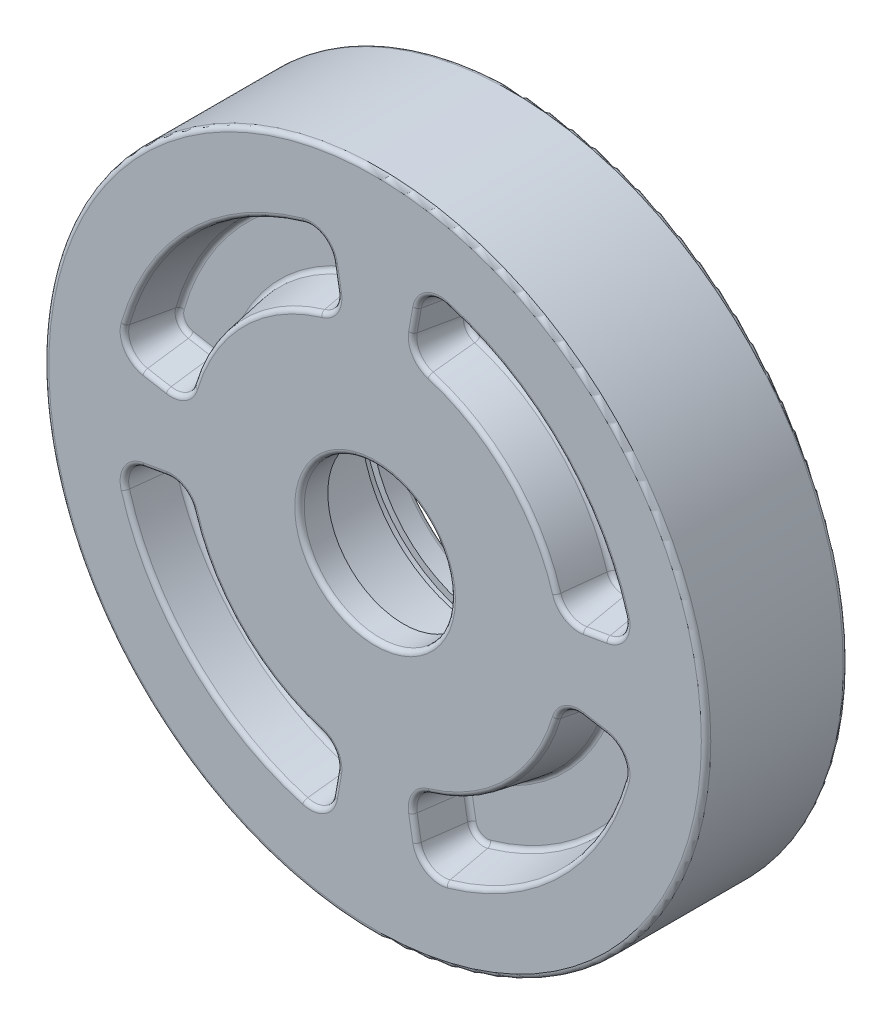
from build123d import *

# Parameters (mm, degrees)
SKETCH1_R                = 70
BOSS_EXTRUDE1_DEPTH      = 15
SKETCH2_R                = 16
CUT_EXTRUDE1_DEPTH       = 6
SKETCH3_R                = 22.5
CUT_EXTRUDE2_DEPTH       = 2
SKETCH4_R                = 26
CUT_EXTRUDE3_DEPTH       = 15
SKETCH5_R                = 27.5
CUT_EXTRUDE4_DEPTH       = 2
SKETCH6_R                = 26
CUT_EXTRUDE5_DEPTH       = 103.102889283
CUT_EXTRUDE6_DEPTH       = 10
CUT_EXTRUDE6_DRAFT       = -10
CIRPATTERN1_COPY_1_DEPTH = 10
CIRPATTERN1_COPY_1_DRAFT = -10
CIRPATTERN1_COPY_2_DEPTH = 10
CIRPATTERN1_COPY_2_DRAFT = -10
CIRPATTERN1_COPY_3_DEPTH = 10
CIRPATTERN1_COPY_3_DRAFT = -10
MIRROR1_COPY_1_DEPTH     = 10
MIRROR1_COPY_1_DRAFT     = -10
MIRROR1_COPY_2_DEPTH     = 10
MIRROR1_COPY_2_DRAFT     = -10
MIRROR1_COPY_3_DEPTH     = 10
MIRROR1_COPY_3_DRAFT     = -10
MIRROR1_COPY_4_DEPTH     = 10
MIRROR1_COPY_4_DRAFT     = -10
FILLET1_R                = 1
FILLET2_R                = 1
SKETCH8_R                = 1.5
CUT_EXTRUDE7_DEPTH       = 10


with BuildPart() as part:
    # Sketch1 → Boss-Extrude1 (new, symmetric)
    with BuildSketch(Plane.XY):
        Circle(SKETCH1_R)
    extrude(amount=BOSS_EXTRUDE1_DEPTH, both=True)

    # Sketch2 → Cut-Extrude1 (cut)
    with BuildSketch(Plane.XY.offset(15)):
        Circle(SKETCH2_R)
    extrude(amount=-CUT_EXTRUDE1_DEPTH, mode=Mode.SUBTRACT)

    # Sketch3 → Cut-Extrude2 (cut)
    with BuildSketch(Plane.XY.offset(9)):
        Circle(SKETCH3_R)
    extrude(amount=-CUT_EXTRUDE2_DEPTH, mode=Mode.SUBTRACT)

    # Sketch4 → Cut-Extrude3 (cut)
    with BuildSketch(Plane.XY.offset(7)):
        Circle(SKETCH4_R)
    extrude(amount=-CUT_EXTRUDE3_DEPTH, mode=Mode.SUBTRACT)

    # Sketch5 → Cut-Extrude4 (cut)
    with BuildSketch(Plane.XY.offset(-8)):
        Circle(SKETCH5_R)
    extrude(amount=-CUT_EXTRUDE4_DEPTH, mode=Mode.SUBTRACT)

    # Sketch6 → Cut-Extrude5 (cut, through all)
    with BuildSketch(Plane.XY.offset(-10)):
        Circle(SKETCH6_R)
    extrude(amount=-CUT_EXTRUDE5_DEPTH, mode=Mode.SUBTRACT)


with BuildPart() as cut_extrude6_tool:
    # Sketch7 → Cut-Extrude6 (with draft: the straight prism first)
    with BuildSketch(Plane(origin=(0, 0, -15), x_dir=(-1, 0, 0), z_dir=(0, 0, -1))):
        with BuildLine():
            ThreePointArc((-8.800542906, 48.942287572), (-11.071183936, 52.316508785), (-15.098039216, 52.887136544))
            ThreePointArc((-15.098039216, 52.887136544), (-38.890872965, 38.890872965), (-52.887136544, 15.098039216))
            ThreePointArc((-52.887136544, 15.098039216), (-52.316508785, 11.071183936), (-48.942287572, 8.800542906))
            Line((-48.942287572, 8.800542906), (-43.987240669, 7.932195568))
            ThreePointArc((-43.987240669, 7.932195568), (-40.494635393, 8.60443107), (-38.3325939, 11.428571429))
            ThreePointArc((-38.3325939, 11.428571429), (-28.284271247, 28.284271247), (-11.428571429, 38.3325939))
            ThreePointArc((-11.428571429, 38.3325939), (-8.60443107, 40.494635393), (-7.932195568, 43.987240669))
            Line((-7.932195568, 43.987240669), (-8.800542906, 48.942287572))
        make_face()
    extrude(amount=-CUT_EXTRUDE6_DEPTH)
    # Cut-Extrude6: the draft: its side faces are tilted about the plane it starts from
    cut_extrude6_sides = [cut_extrude6_tool.faces().sort_by_distance(p)[0] for p in [
        (8.60443107, 40.494635393, -10),
        (8.366369237, 46.46476412, -10),
        (11.071183936, 52.316508785, -10),
        (38.890872965, 38.890872965, -10),
        (52.316508785, 11.071183936, -10),
        (46.46476412, 8.366369237, -10),
        (40.494635393, 8.60443107, -10),
        (28.284271247, 28.284271247, -10),
    ]]
    draft(cut_extrude6_sides, Plane(origin=(0, 0, -15), x_dir=(-1, 0, 0), z_dir=(0, 0, -1)), CUT_EXTRUDE6_DRAFT)


with BuildPart() as part_1:
    add(part.part)

    # Cut-Extrude6: cut by cut_extrude6_tool
    add(cut_extrude6_tool.part, mode=Mode.SUBTRACT)


with BuildPart() as cirpattern1_copy_1_tool:
    # CirPattern1 copy 1 sketch → CirPattern1 copy 1 (with draft: the straight prism first)
    with BuildSketch(Plane(origin=(0, 0, -15), x_dir=(0, -1, 0), z_dir=(0, 0, -1))):
        with BuildLine():
            ThreePointArc((-8.800542906, 48.942287572), (-11.071183936, 52.316508785), (-15.098039216, 52.887136544))
            ThreePointArc((-15.098039216, 52.887136544), (-38.890872965, 38.890872965), (-52.887136544, 15.098039216))
            ThreePointArc((-52.887136544, 15.098039216), (-52.316508785, 11.071183936), (-48.942287572, 8.800542906))
            Line((-48.942287572, 8.800542906), (-43.987240669, 7.932195568))
            ThreePointArc((-43.987240669, 7.932195568), (-40.494635393, 8.60443107), (-38.3325939, 11.428571429))
            ThreePointArc((-38.3325939, 11.428571429), (-28.284271247, 28.284271247), (-11.428571429, 38.3325939))
            ThreePointArc((-11.428571429, 38.3325939), (-8.60443107, 40.494635393), (-7.932195568, 43.987240669))
            Line((-7.932195568, 43.987240669), (-8.800542906, 48.942287572))
        make_face()
    extrude(amount=-CIRPATTERN1_COPY_1_DEPTH)
    # CirPattern1 copy 1: the draft: its side faces are tilted about the plane it starts from
    cirpattern1_copy_1_sides = [cirpattern1_copy_1_tool.faces().sort_by_distance(p)[0] for p in [
        (-40.494635393, 8.60443107, -10),
        (-46.46476412, 8.366369237, -10),
        (-52.316508785, 11.071183936, -10),
        (-38.890872965, 38.890872965, -10),
        (-11.071183936, 52.316508785, -10),
        (-8.366369237, 46.46476412, -10),
        (-8.60443107, 40.494635393, -10),
        (-28.284271247, 28.284271247, -10),
    ]]
    draft(cirpattern1_copy_1_sides, Plane(origin=(0, 0, -15), x_dir=(0, -1, 0), z_dir=(0, 0, -1)), CIRPATTERN1_COPY_1_DRAFT)


with BuildPart() as part_2:
    add(part_1.part)

    # CirPattern1 copy 1: cut by cirpattern1_copy_1_tool
    add(cirpattern1_copy_1_tool.part, mode=Mode.SUBTRACT)


with BuildPart() as cirpattern1_copy_2_tool:
    # CirPattern1 copy 2 sketch → CirPattern1 copy 2 (with draft: the straight prism first)
    with BuildSketch(Plane(origin=(0, 0, -15), x_dir=(1, 0, 0), z_dir=(0, 0, -1))):
        with BuildLine():
            ThreePointArc((-8.800542906, 48.942287572), (-11.071183936, 52.316508785), (-15.098039216, 52.887136544))
            ThreePointArc((-15.098039216, 52.887136544), (-38.890872965, 38.890872965), (-52.887136544, 15.098039216))
            ThreePointArc((-52.887136544, 15.098039216), (-52.316508785, 11.071183936), (-48.942287572, 8.800542906))
            Line((-48.942287572, 8.800542906), (-43.987240669, 7.932195568))
            ThreePointArc((-43.987240669, 7.932195568), (-40.494635393, 8.60443107), (-38.3325939, 11.428571429))
            ThreePointArc((-38.3325939, 11.428571429), (-28.284271247, 28.284271247), (-11.428571429, 38.3325939))
            ThreePointArc((-11.428571429, 38.3325939), (-8.60443107, 40.494635393), (-7.932195568, 43.987240669))
            Line((-7.932195568, 43.987240669), (-8.800542906, 48.942287572))
        make_face()
    extrude(amount=-CIRPATTERN1_COPY_2_DEPTH)
    # CirPattern1 copy 2: the draft: its side faces are tilted about the plane it starts from
    cirpattern1_copy_2_sides = [cirpattern1_copy_2_tool.faces().sort_by_distance(p)[0] for p in [
        (-8.60443107, -40.494635393, -10),
        (-8.366369237, -46.46476412, -10),
        (-11.071183936, -52.316508785, -10),
        (-38.890872965, -38.890872965, -10),
        (-52.316508785, -11.071183936, -10),
        (-46.46476412, -8.366369237, -10),
        (-40.494635393, -8.60443107, -10),
        (-28.284271247, -28.284271247, -10),
    ]]
    draft(cirpattern1_copy_2_sides, Plane(origin=(0, 0, -15), x_dir=(1, 0, 0), z_dir=(0, 0, -1)), CIRPATTERN1_COPY_2_DRAFT)


with BuildPart() as part_3:
    add(part_2.part)

    # CirPattern1 copy 2: cut by cirpattern1_copy_2_tool
    add(cirpattern1_copy_2_tool.part, mode=Mode.SUBTRACT)


with BuildPart() as cirpattern1_copy_3_tool:
    # CirPattern1 copy 3 sketch → CirPattern1 copy 3 (with draft: the straight prism first)
    with BuildSketch(Plane.YX.offset(15)):
        with BuildLine():
            ThreePointArc((-8.800542906, 48.942287572), (-11.071183936, 52.316508785), (-15.098039216, 52.887136544))
            ThreePointArc((-15.098039216, 52.887136544), (-38.890872965, 38.890872965), (-52.887136544, 15.098039216))
            ThreePointArc((-52.887136544, 15.098039216), (-52.316508785, 11.071183936), (-48.942287572, 8.800542906))
            Line((-48.942287572, 8.800542906), (-43.987240669, 7.932195568))
            ThreePointArc((-43.987240669, 7.932195568), (-40.494635393, 8.60443107), (-38.3325939, 11.428571429))
            ThreePointArc((-38.3325939, 11.428571429), (-28.284271247, 28.284271247), (-11.428571429, 38.3325939))
            ThreePointArc((-11.428571429, 38.3325939), (-8.60443107, 40.494635393), (-7.932195568, 43.987240669))
            Line((-7.932195568, 43.987240669), (-8.800542906, 48.942287572))
        make_face()
    extrude(amount=-CIRPATTERN1_COPY_3_DEPTH)
    # CirPattern1 copy 3: the draft: its side faces are tilted about the plane it starts from
    cirpattern1_copy_3_sides = [cirpattern1_copy_3_tool.faces().sort_by_distance(p)[0] for p in [
        (40.494635393, -8.60443107, -10),
        (46.46476412, -8.366369237, -10),
        (52.316508785, -11.071183936, -10),
        (38.890872965, -38.890872965, -10),
        (11.071183936, -52.316508785, -10),
        (8.366369237, -46.46476412, -10),
        (8.60443107, -40.494635393, -10),
        (28.284271247, -28.284271247, -10),
    ]]
    draft(cirpattern1_copy_3_sides, Plane.YX.offset(15), CIRPATTERN1_COPY_3_DRAFT)


with BuildPart() as part_4:
    add(part_3.part)

    # CirPattern1 copy 3: cut by cirpattern1_copy_3_tool
    add(cirpattern1_copy_3_tool.part, mode=Mode.SUBTRACT)


with BuildPart() as mirror1_copy_1_tool:
    # Mirror1 copy 1 sketch → Mirror1 copy 1 (with draft: the straight prism first)
    with BuildSketch(Plane(origin=(0, 0, 15), x_dir=(-1, 0, 0), z_dir=(0, 0, 1))):
        with BuildLine():
            ThreePointArc((-8.800542906, -48.942287572), (-11.071183936, -52.316508785), (-15.098039216, -52.887136544))
            ThreePointArc((-15.098039216, -52.887136544), (-38.890872965, -38.890872965), (-52.887136544, -15.098039216))
            ThreePointArc((-52.887136544, -15.098039216), (-52.316508785, -11.071183936), (-48.942287572, -8.800542906))
            Line((-48.942287572, -8.800542906), (-43.987240669, -7.932195568))
            ThreePointArc((-43.987240669, -7.932195568), (-40.494635393, -8.60443107), (-38.3325939, -11.428571429))
            ThreePointArc((-38.3325939, -11.428571429), (-28.284271247, -28.284271247), (-11.428571429, -38.3325939))
            ThreePointArc((-11.428571429, -38.3325939), (-8.60443107, -40.494635393), (-7.932195568, -43.987240669))
            Line((-7.932195568, -43.987240669), (-8.800542906, -48.942287572))
        make_face()
    extrude(amount=-MIRROR1_COPY_1_DEPTH)
    # Mirror1 copy 1: the draft: its side faces are tilted about the plane it starts from
    mirror1_copy_1_sides = [mirror1_copy_1_tool.faces().sort_by_distance(p)[0] for p in [
        (8.60443107, 40.494635393, 10),
        (8.366369237, 46.46476412, 10),
        (11.071183936, 52.316508785, 10),
        (38.890872965, 38.890872965, 10),
        (52.316508785, 11.071183936, 10),
        (46.46476412, 8.366369237, 10),
        (40.494635393, 8.60443107, 10),
        (28.284271247, 28.284271247, 10),
    ]]
    draft(mirror1_copy_1_sides, Plane(origin=(0, 0, 15), x_dir=(-1, 0, 0), z_dir=(0, 0, 1)), MIRROR1_COPY_1_DRAFT)


with BuildPart() as part_5:
    add(part_4.part)

    # Mirror1 copy 1: cut by mirror1_copy_1_tool
    add(mirror1_copy_1_tool.part, mode=Mode.SUBTRACT)


with BuildPart() as mirror1_copy_2_tool:
    # Mirror1 copy 2 sketch → Mirror1 copy 2 (with draft: the straight prism first)
    with BuildSketch(Plane(origin=(0, 0, 15), x_dir=(0, -1, 0), z_dir=(0, 0, 1))):
        with BuildLine():
            ThreePointArc((-8.800542906, -48.942287572), (-11.071183936, -52.316508785), (-15.098039216, -52.887136544))
            ThreePointArc((-15.098039216, -52.887136544), (-38.890872965, -38.890872965), (-52.887136544, -15.098039216))
            ThreePointArc((-52.887136544, -15.098039216), (-52.316508785, -11.071183936), (-48.942287572, -8.800542906))
            Line((-48.942287572, -8.800542906), (-43.987240669, -7.932195568))
            ThreePointArc((-43.987240669, -7.932195568), (-40.494635393, -8.60443107), (-38.3325939, -11.428571429))
            ThreePointArc((-38.3325939, -11.428571429), (-28.284271247, -28.284271247), (-11.428571429, -38.3325939))
            ThreePointArc((-11.428571429, -38.3325939), (-8.60443107, -40.494635393), (-7.932195568, -43.987240669))
            Line((-7.932195568, -43.987240669), (-8.800542906, -48.942287572))
        make_face()
    extrude(amount=-MIRROR1_COPY_2_DEPTH)
    # Mirror1 copy 2: the draft: its side faces are tilted about the plane it starts from
    mirror1_copy_2_sides = [mirror1_copy_2_tool.faces().sort_by_distance(p)[0] for p in [
        (-40.494635393, 8.60443107, 10),
        (-46.46476412, 8.366369237, 10),
        (-52.316508785, 11.071183936, 10),
        (-38.890872965, 38.890872965, 10),
        (-11.071183936, 52.316508785, 10),
        (-8.366369237, 46.46476412, 10),
        (-8.60443107, 40.494635393, 10),
        (-28.284271247, 28.284271247, 10),
    ]]
    draft(mirror1_copy_2_sides, Plane(origin=(0, 0, 15), x_dir=(0, -1, 0), z_dir=(0, 0, 1)), MIRROR1_COPY_2_DRAFT)


with BuildPart() as part_6:
    add(part_5.part)

    # Mirror1 copy 2: cut by mirror1_copy_2_tool
    add(mirror1_copy_2_tool.part, mode=Mode.SUBTRACT)


with BuildPart() as mirror1_copy_3_tool:
    # Mirror1 copy 3 sketch → Mirror1 copy 3 (with draft: the straight prism first)
    with BuildSketch(Plane.XY.offset(15)):
        with BuildLine():
            ThreePointArc((-8.800542906, -48.942287572), (-11.071183936, -52.316508785), (-15.098039216, -52.887136544))
            ThreePointArc((-15.098039216, -52.887136544), (-38.890872965, -38.890872965), (-52.887136544, -15.098039216))
            ThreePointArc((-52.887136544, -15.098039216), (-52.316508785, -11.071183936), (-48.942287572, -8.800542906))
            Line((-48.942287572, -8.800542906), (-43.987240669, -7.932195568))
            ThreePointArc((-43.987240669, -7.932195568), (-40.494635393, -8.60443107), (-38.3325939, -11.428571429))
            ThreePointArc((-38.3325939, -11.428571429), (-28.284271247, -28.284271247), (-11.428571429, -38.3325939))
            ThreePointArc((-11.428571429, -38.3325939), (-8.60443107, -40.494635393), (-7.932195568, -43.987240669))
            Line((-7.932195568, -43.987240669), (-8.800542906, -48.942287572))
        make_face()
    extrude(amount=-MIRROR1_COPY_3_DEPTH)
    # Mirror1 copy 3: the draft: its side faces are tilted about the plane it starts from
    mirror1_copy_3_sides = [mirror1_copy_3_tool.faces().sort_by_distance(p)[0] for p in [
        (-8.60443107, -40.494635393, 10),
        (-8.366369237, -46.46476412, 10),
        (-11.071183936, -52.316508785, 10),
        (-38.890872965, -38.890872965, 10),
        (-52.316508785, -11.071183936, 10),
        (-46.46476412, -8.366369237, 10),
        (-40.494635393, -8.60443107, 10),
        (-28.284271247, -28.284271247, 10),
    ]]
    draft(mirror1_copy_3_sides, Plane.XY.offset(15), MIRROR1_COPY_3_DRAFT)


with BuildPart() as part_7:
    add(part_6.part)

    # Mirror1 copy 3: cut by mirror1_copy_3_tool
    add(mirror1_copy_3_tool.part, mode=Mode.SUBTRACT)


with BuildPart() as mirror1_copy_4_tool:
    # Mirror1 copy 4 sketch → Mirror1 copy 4 (with draft: the straight prism first)
    with BuildSketch(Plane(origin=(0, 0, 15), x_dir=(0, 1, 0), z_dir=(0, 0, 1))):
        with BuildLine():
            ThreePointArc((-8.800542906, -48.942287572), (-11.071183936, -52.316508785), (-15.098039216, -52.887136544))
            ThreePointArc((-15.098039216, -52.887136544), (-38.890872965, -38.890872965), (-52.887136544, -15.098039216))
            ThreePointArc((-52.887136544, -15.098039216), (-52.316508785, -11.071183936), (-48.942287572, -8.800542906))
            Line((-48.942287572, -8.800542906), (-43.987240669, -7.932195568))
            ThreePointArc((-43.987240669, -7.932195568), (-40.494635393, -8.60443107), (-38.3325939, -11.428571429))
            ThreePointArc((-38.3325939, -11.428571429), (-28.284271247, -28.284271247), (-11.428571429, -38.3325939))
            ThreePointArc((-11.428571429, -38.3325939), (-8.60443107, -40.494635393), (-7.932195568, -43.987240669))
            Line((-7.932195568, -43.987240669), (-8.800542906, -48.942287572))
        make_face()
    extrude(amount=-MIRROR1_COPY_4_DEPTH)
    # Mirror1 copy 4: the draft: its side faces are tilted about the plane it starts from
    mirror1_copy_4_sides = [mirror1_copy_4_tool.faces().sort_by_distance(p)[0] for p in [
        (40.494635393, -8.60443107, 10),
        (46.46476412, -8.366369237, 10),
        (52.316508785, -11.071183936, 10),
        (38.890872965, -38.890872965, 10),
        (11.071183936, -52.316508785, 10),
        (8.366369237, -46.46476412, 10),
        (8.60443107, -40.494635393, 10),
        (28.284271247, -28.284271247, 10),
    ]]
    draft(mirror1_copy_4_sides, Plane(origin=(0, 0, 15), x_dir=(0, 1, 0), z_dir=(0, 0, 1)), MIRROR1_COPY_4_DRAFT)


with BuildPart() as part_8:
    add(part_7.part)

    # Mirror1 copy 4: cut by mirror1_copy_4_tool
    add(mirror1_copy_4_tool.part, mode=Mode.SUBTRACT)

    # Fillet1
    fillet1_edges = [part_8.edges().sort_by_distance(p)[0] for p in [
        (-70, 0, -15),
        (-26, 0, -15),
        (10.104166728, 41.421950532, -5),
        (29.531091285, 29.531091285, -5),
        (41.421950532, 10.104166728, -5),
        (46.160398173, 10.103171408, -5),
        (50.82221036, 12.007235554, -5),
        (37.644052928, 37.644052928, -5),
        (12.007235554, 50.82221036, -5),
        (10.103171408, 46.160398173, -5),
        (8.60443107, 40.494635393, -15),
        (8.366369237, 46.46476412, -15),
        (11.071183936, 52.316508785, -15),
        (38.890872965, 38.890872965, -15),
        (52.316508785, 11.071183936, -15),
        (46.46476412, 8.366369237, -15),
        (40.494635393, 8.60443107, -15),
        (28.284271247, 28.284271247, -15),
        (41.421950532, -10.104166728, -5),
        (29.531091285, -29.531091285, -5),
        (10.104166728, -41.421950532, -5),
        (10.103171408, -46.160398173, -5),
        (12.007235554, -50.82221036, -5),
        (37.644052928, -37.644052928, -5),
        (50.82221036, -12.007235554, -5),
        (46.160398173, -10.103171408, -5),
        (40.494635393, -8.60443107, -15),
        (46.46476412, -8.366369237, -15),
        (52.316508785, -11.071183936, -15),
        (38.890872965, -38.890872965, -15),
        (11.071183936, -52.316508785, -15),
        (8.366369237, -46.46476412, -15),
        (8.60443107, -40.494635393, -15),
        (28.284271247, -28.284271247, -15),
        (-10.104166728, -41.421950532, -5),
        (-29.531091285, -29.531091285, -5),
        (-41.421950532, -10.104166728, -5),
        (-46.160398173, -10.103171408, -5),
        (-50.82221036, -12.007235554, -5),
        (-37.644052928, -37.644052928, -5),
        (-12.007235554, -50.82221036, -5),
        (-10.103171408, -46.160398173, -5),
        (-8.60443107, -40.494635393, -15),
        (-8.366369237, -46.46476412, -15),
        (-11.071183936, -52.316508785, -15),
        (-38.890872965, -38.890872965, -15),
        (-52.316508785, -11.071183936, -15),
        (-46.46476412, -8.366369237, -15),
        (-40.494635393, -8.60443107, -15),
        (-28.284271247, -28.284271247, -15),
        (-41.421950532, 10.104166728, -5),
        (-29.531091285, 29.531091285, -5),
        (-10.104166728, 41.421950532, -5),
        (-10.103171408, 46.160398173, -5),
        (-12.007235554, 50.82221036, -5),
        (-37.644052928, 37.644052928, -5),
        (-50.82221036, 12.007235554, -5),
        (-46.160398173, 10.103171408, -5),
        (-40.494635393, 8.60443107, -15),
        (-46.46476412, 8.366369237, -15),
        (-52.316508785, 11.071183936, -15),
        (-38.890872965, 38.890872965, -15),
        (-11.071183936, 52.316508785, -15),
        (-8.366369237, 46.46476412, -15),
        (-8.60443107, 40.494635393, -15),
        (-28.284271247, 28.284271247, -15),
    ]]
    fillet(fillet1_edges, radius=FILLET1_R)

    # Fillet2
    fillet2_edges = [part_8.edges().sort_by_distance(p)[0] for p in [
        (8.60443107, 40.494635393, 15),
        (8.366369237, 46.46476412, 15),
        (11.071183936, 52.316508785, 15),
        (38.890872965, 38.890872965, 15),
        (52.316508785, 11.071183936, 15),
        (46.46476412, 8.366369237, 15),
        (40.494635393, 8.60443107, 15),
        (28.284271247, 28.284271247, 15),
        (10.104166728, 41.421950532, 5),
        (10.103171408, 46.160398173, 5),
        (12.007235554, 50.82221036, 5),
        (37.644052928, 37.644052928, 5),
        (50.82221036, 12.007235554, 5),
        (46.160398173, 10.103171408, 5),
        (41.421950532, 10.104166728, 5),
        (29.531091285, 29.531091285, 5),
        (40.494635393, -8.60443107, 15),
        (46.46476412, -8.366369237, 15),
        (52.316508785, -11.071183936, 15),
        (38.890872965, -38.890872965, 15),
        (11.071183936, -52.316508785, 15),
        (8.366369237, -46.46476412, 15),
        (8.60443107, -40.494635393, 15),
        (28.284271247, -28.284271247, 15),
        (41.421950532, -10.104166728, 5),
        (46.160398173, -10.103171408, 5),
        (50.82221036, -12.007235554, 5),
        (37.644052928, -37.644052928, 5),
        (12.007235554, -50.82221036, 5),
        (10.103171408, -46.160398173, 5),
        (10.104166728, -41.421950532, 5),
        (29.531091285, -29.531091285, 5),
        (-8.60443107, -40.494635393, 15),
        (-8.366369237, -46.46476412, 15),
        (-11.071183936, -52.316508785, 15),
        (-38.890872965, -38.890872965, 15),
        (-52.316508785, -11.071183936, 15),
        (-46.46476412, -8.366369237, 15),
        (-40.494635393, -8.60443107, 15),
        (-28.284271247, -28.284271247, 15),
        (-10.104166728, -41.421950532, 5),
        (-10.103171408, -46.160398173, 5),
        (-12.007235554, -50.82221036, 5),
        (-37.644052928, -37.644052928, 5),
        (-50.82221036, -12.007235554, 5),
        (-46.160398173, -10.103171408, 5),
        (-41.421950532, -10.104166728, 5),
        (-29.531091285, -29.531091285, 5),
        (-40.494635393, 8.60443107, 15),
        (-46.46476412, 8.366369237, 15),
        (-52.316508785, 11.071183936, 15),
        (-38.890872965, 38.890872965, 15),
        (-11.071183936, 52.316508785, 15),
        (-8.366369237, 46.46476412, 15),
        (-8.60443107, 40.494635393, 15),
        (-28.284271247, 28.284271247, 15),
        (-41.421950532, 10.104166728, 5),
        (-46.160398173, 10.103171408, 5),
        (-50.82221036, 12.007235554, 5),
        (-37.644052928, 37.644052928, 5),
        (-12.007235554, 50.82221036, 5),
        (-10.103171408, 46.160398173, 5),
        (-10.104166728, 41.421950532, 5),
        (-29.531091285, 29.531091285, 5),
        (-70, 0, 15),
        (-16, 0, 15),
    ]]
    fillet(fillet2_edges, radius=FILLET2_R)

    # Sketch8 → Cut-Extrude7 (cut)
    with BuildSketch(Plane(origin=(0, 0, -15), x_dir=(-1, 0, 0), z_dir=(0, 0, -1))):
        with Locations((0, 32.5)):
            Circle(SKETCH8_R)
        with Locations((28.145825623, -16.25)):
            Circle(SKETCH8_R)
        with Locations((-28.145825623, -16.25)):
            Circle(SKETCH8_R)
    extrude(amount=-CUT_EXTRUDE7_DEPTH, mode=Mode.SUBTRACT)


solid = part_8.part
